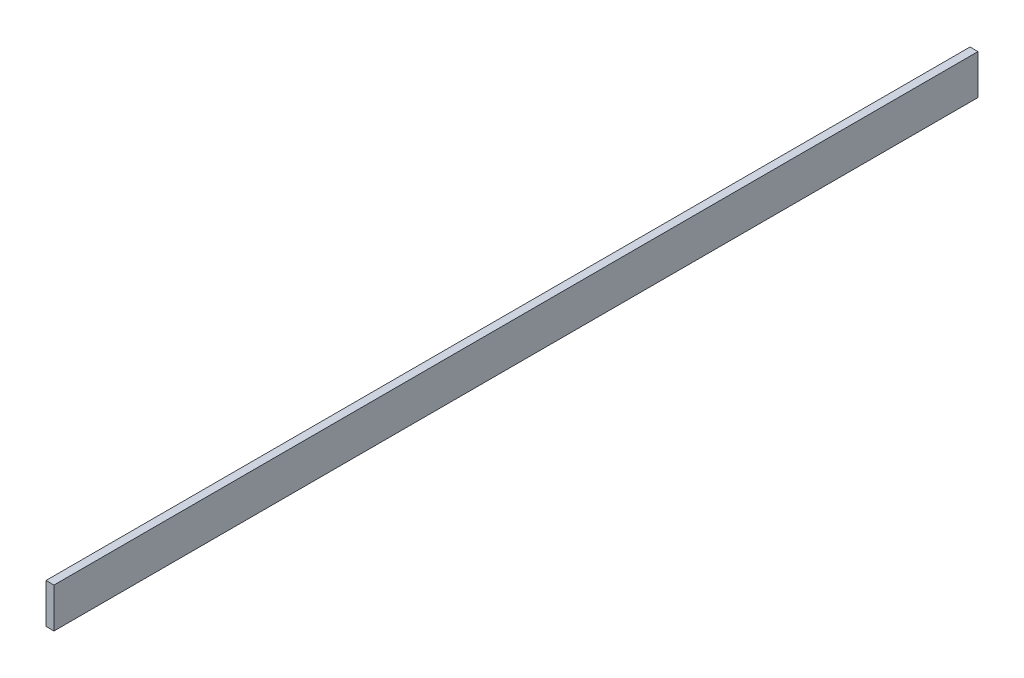
SolidWorks part; units mm, degrees
ref_plane "Front Plane" through (0, 0, 0) normal (0, 0, 1) x (1, 0, 0)
ref_plane "Top Plane" through (0, 0, 0) normal (0, 1, 0) x (1, 0, 0)
ref_plane "Right Plane" through (0, 0, 0) normal (1, 0, 0) x (0, 0, -1)
sketch "Sketch1" plane through (0, 0, 0) normal (0, 0, 1) x (1, 0, 0)
  line L1 (0, 0) -> (5, 0)
  line L2 (0, 0) -> (0, 25)
  line L3 (0, 25) -> (5, 25)
  line L4 (5, 0) -> (5, 25)
  dimension "D1" = 25
  dimension "D2" = 5
extrude "Boss-Extrude1" add sketch "Sketch1" along normal blind 580
